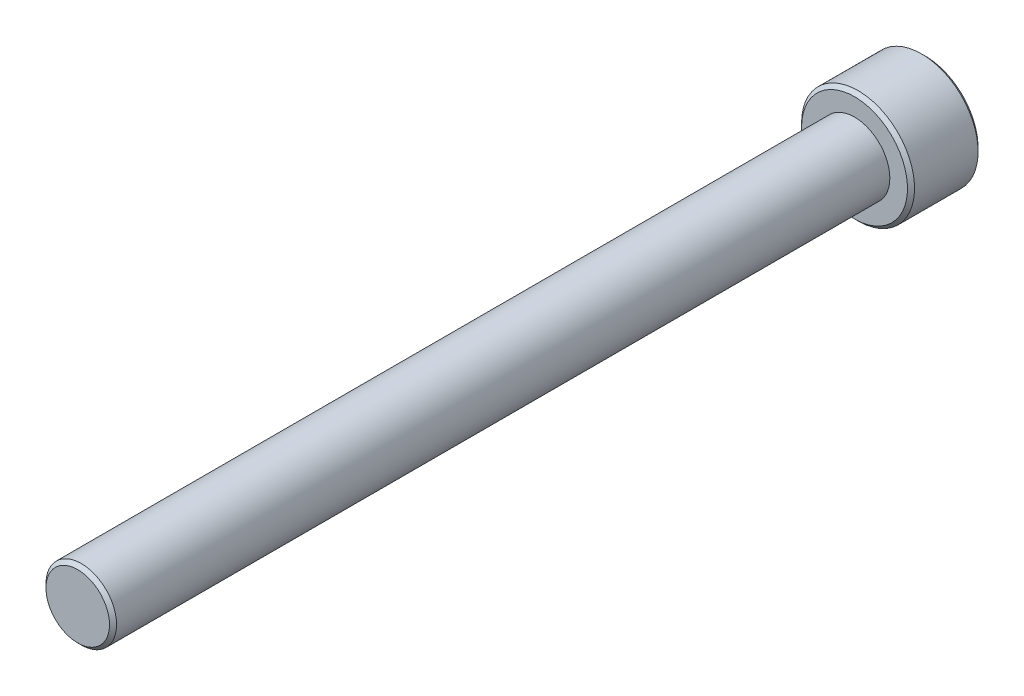
SolidWorks part; units mm, degrees
material "Q235B"
ref_plane "Front Plane" through (0, 0, 0) normal (0, 0, 1) x (1, 0, 0)
ref_plane "Top Plane" through (0, 0, 0) normal (0, 1, 0) x (1, 0, 0)
ref_plane "Right Plane" through (0, 0, 0) normal (1, 0, 0) x (0, 0, -1)
sketch "Sketch1" plane through (0, 0, 0) normal (0, 0, 1) x (1, 0, 0)
  circle A1 centre (0, 0) radius 5
  dimension "D2" = 10
extrude "Boss-Extrude1" add sketch "Sketch1" along normal blind 110
sketch "Sketch2" plane through (0, 0, 0) normal (0, 0, -1) x (-1, 0, 0)
  circle A0 centre (0, 0) radius 8
  dimension "D1" = 16
extrude "Boss-Extrude2" add sketch "Sketch2" along normal blind 10
chamfer "Chamfer1" distance 0.5 angle 45 3 edges at (5, 0, 110) (-8, 0, -10) (-8, 0, 0)
